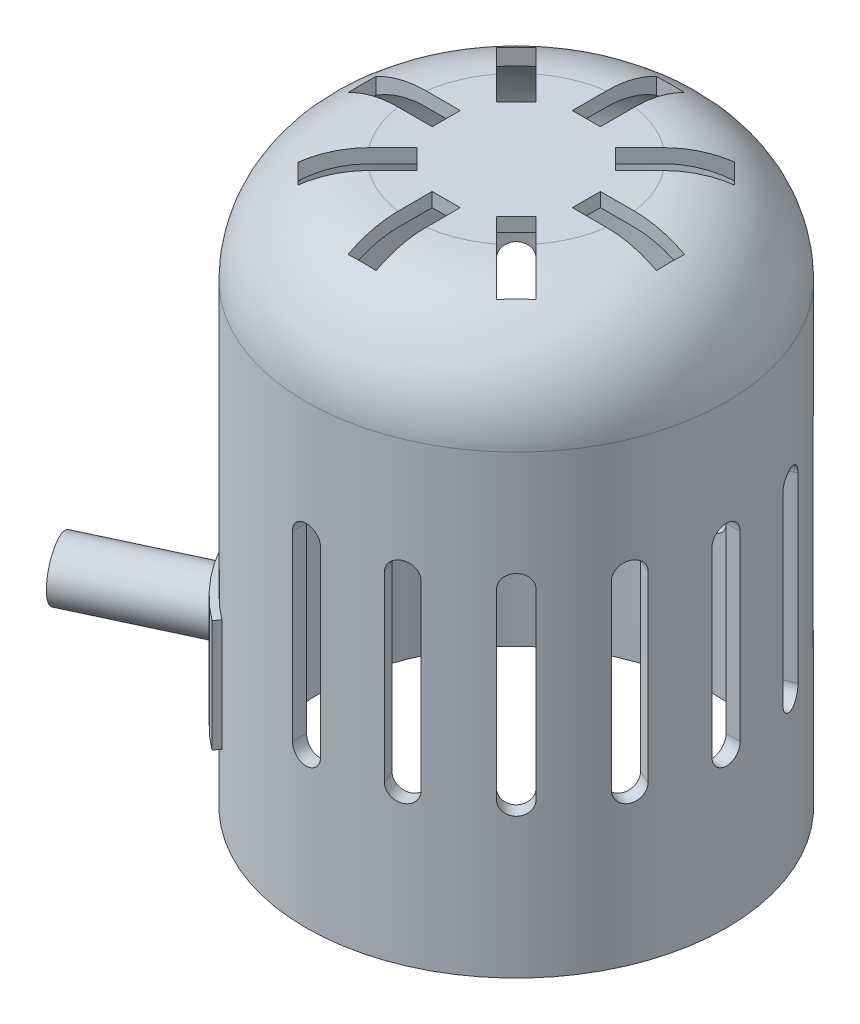
from build123d import *

# Parameters (mm, degrees)
SKETCH1_R           = 30
BOSS_EXTRUDE3_DEPTH = 80
FILLET3_R           = 15
SHELL3_T            = -2
SKETCH3_W           = 4
SKETCH3_H           = 12
SKETCH3_W_2         = 12
SKETCH3_H_2         = 4
CUT_EXTRUDE4_DEPTH  = 10
CUT_EXTRUDE5_DEPTH  = 66
CIRPATTERN1_COUNT   = 16
BOSS_EXTRUDE4_DEPTH = 16
SKETCH16_R          = 4
BOSS_EXTRUDE5_DEPTH = 18


with BuildPart() as part:
    # Sketch1 → Boss-Extrude3 (new body)
    with BuildSketch(Plane(origin=(0, 0, 0), x_dir=(1, 0, 0), z_dir=(0, 1, 0))):
        with Locations(Location((0, 0, 0), (0, 0, 270))):
            Circle(SKETCH1_R)
    extrude(amount=BOSS_EXTRUDE3_DEPTH)

    # Fillet3
    fillet3_edges = [part.edges().sort_by_distance(p)[0] for p in [
        (0, 80, -30),
    ]]
    fillet(fillet3_edges, radius=FILLET3_R)

    # Shell3
    shell3_openings = [part.faces().sort_by_distance(p)[0] for p in [
        (0, 0, 0),
    ]]
    offset(amount=SHELL3_T, openings=shell3_openings, kind=Kind.INTERSECTION)

    # Sketch3 → Cut-Extrude4 (cut, symmetric)
    with BuildSketch(Plane(origin=(0, 78, 0), x_dir=(1, 0, 0), z_dir=(0, 1, 0))):
        Polygon((14.142135624, 16.970562748), (16.970562748, 14.142135624), (8.485281374, 5.656854249), (5.656854249, 8.485281374), align=None)
        with Locations((0, 16)):
            Rectangle(SKETCH3_W, SKETCH3_H)
        with Locations((16, 0)):
            Rectangle(SKETCH3_W_2, SKETCH3_H_2)
        Polygon((16.970562748, -14.142135624), (14.142135624, -16.970562748), (5.656854249, -8.485281374), (8.485281374, -5.656854249), align=None)
        with Locations((0, -16)):
            Rectangle(SKETCH3_W, SKETCH3_H)
        Polygon((-14.142135624, -16.970562748), (-16.970562748, -14.142135624), (-8.485281374, -5.656854249), (-5.656854249, -8.485281374), align=None)
        with Locations((-16, 0)):
            Rectangle(SKETCH3_W_2, SKETCH3_H_2)
        Polygon((-16.970562748, 14.142135624), (-14.142135624, 16.970562748), (-5.656854249, 8.485281374), (-8.485281374, 5.656854249), align=None)
    extrude(amount=CUT_EXTRUDE4_DEPTH, both=True, mode=Mode.SUBTRACT)

    # Sketch4 → Cut-Extrude5 (cut)
    with BuildSketch(Plane.XY):
        with BuildLine():
            Line((2, 48), (2, 22))
            ThreePointArc((2, 22), (0, 20), (-2, 22))
            Line((-2, 22), (-2, 48))
            ThreePointArc((-2, 48), (0, 50), (2, 48))
        make_face()
    cut_extrude5 = extrude(amount=-CUT_EXTRUDE5_DEPTH, mode=Mode.SUBTRACT)

    # CirPattern1: Cut-Extrude5 ×16 about axis, 5 skipped
    cirpattern1_axis = Axis((0, 0, 0), (0, 1, 0))
    add([cut_extrude5.rotate(cirpattern1_axis, i * 360 / CIRPATTERN1_COUNT) for i in range(1, CIRPATTERN1_COUNT) if i not in (3, 4, 5, 6, 7)], mode=Mode.SUBTRACT)

    # Sketch15 → Boss-Extrude4 (add)
    with BuildSketch(Plane(origin=(0, 10, 0), x_dir=(-1, 0, 0), z_dir=(0, -1, 0))):
        with BuildLine():
            Line((29.962317741, 1.503168507), (30.961061666, 1.553274124))
            ThreePointArc((30.961061666, 1.553274124), (28.086325113, -13.120912378), (18.676743596, -24.742256337))
            Line((18.676743596, -24.742256337), (18.074267996, -23.944119036))
            ThreePointArc((18.074267996, -23.944119036), (27.180314626, -12.69765714), (29.962317741, 1.503168507))
        make_face()
    extrude(amount=-BOSS_EXTRUDE4_DEPTH)


with BuildPart() as body_2:
    # Sketch16 → Boss-Extrude5 (new body)
    with BuildSketch(Plane(origin=(-28.095541398, 0, 13.101166114), x_dir=(0, -1, 0), z_dir=(-0.906307787036651, 0, 0.4226182617406972))):
        with Locations(Location((-17.587533018, 0, 0), (0, 0, 90))):
            Circle(SKETCH16_R)
    extrude(amount=BOSS_EXTRUDE5_DEPTH)


solid = Compound([part.part, body_2.part])
